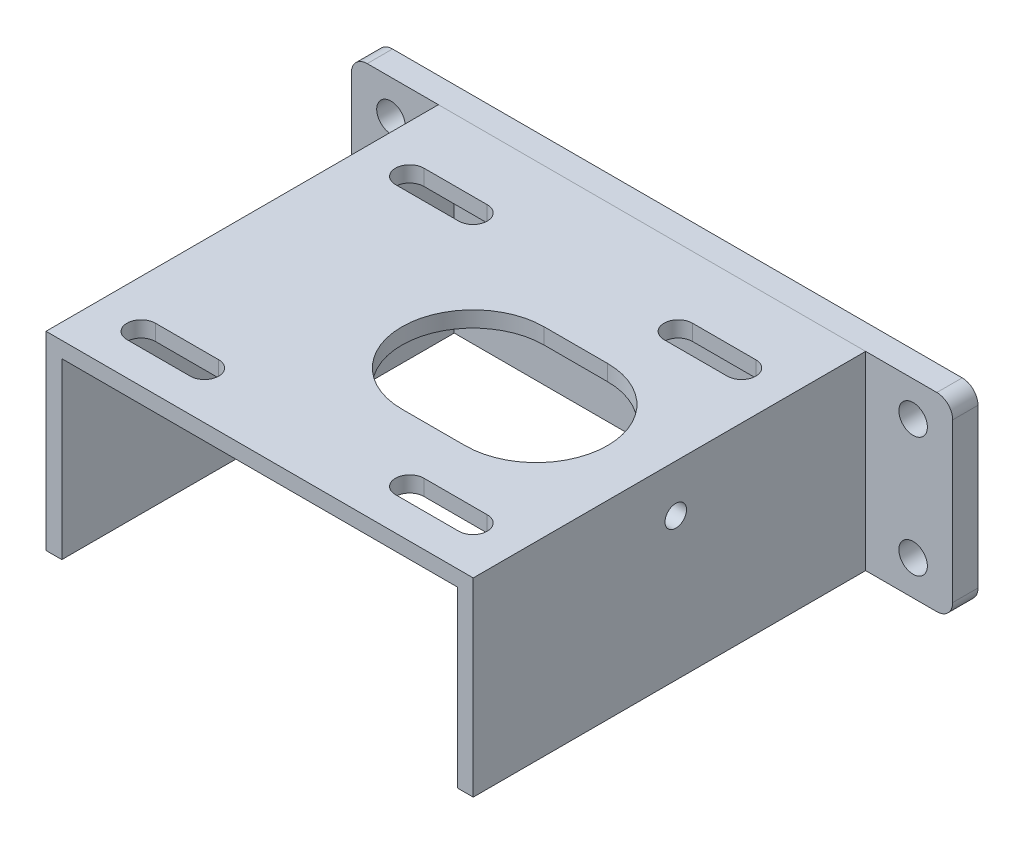
SolidWorks part; units mm, degrees
ref_plane "前视基准面" through (0, 0, 0) normal (0, 0, 1) x (1, 0, 0)
ref_plane "上视基准面" through (0, 0, 0) normal (0, 1, 0) x (1, 0, 0)
ref_plane "右视基准面" through (0, 0, 0) normal (1, 0, 0) x (0, 0, -1)
sketch "草图1" plane through (0, 0, 0) normal (0, 0, 1) x (1, 0, 0)
  line L1 (-95, 30) -> (95, 30)
  line L2 (-95, 30) -> (-95, -30)
  line L3 (-95, -30) -> (95, -30)
  line L4 (95, 30) -> (95, -30)
  line L5 (-95, 30) -> (95, -30) construction
  line L6 (-95, -30) -> (95, 30) construction
  point P0 (0, 0)
  dimension "D1" = 60
  dimension "D2" = 190
extrude "凸台-拉伸1" add sketch "草图1" along normal blind 8
sketch "草图2" plane through (0, 0, 8) normal (0, 0, 1) x (1, 0, 0)
  line L6 (-82.5, 19) -> (82.5, 19) construction
  line L7 (-82.5, 19) -> (-82.5, -19) construction
  line L8 (-82.5, -19) -> (82.5, -19) construction
  line L9 (82.5, 19) -> (82.5, -19) construction
  line L10 (-82.5, 19) -> (82.5, -19) construction
  line L11 (-82.5, -19) -> (82.5, 19) construction
  circle A0 centre (-82.5, 19) radius 4.5
  circle A1 centre (82.5, 19) radius 4.5
  circle A2 centre (82.5, -19) radius 4.5
  circle A3 centre (-82.5, -19) radius 4.5
  point P0 (0, 0)
  dimension "D3" = 9
  dimension "D1" = 165
  dimension "D2" = 38
extrude "切除-拉伸1" cut sketch "草图2" against normal blind 8
sketch "草图3" plane through (0, 0, 8) normal (0, 0, 1) x (1, 0, 0)
  line L0 (-67.5, 30) -> (-67.5, -30)
  line L1 (95, 30) -> (-95, 30) construction
  line L2 (-95, -30) -> (95, -30) construction
  line L3 (-67.5, -30) -> (-62.5, -30)
  line L4 (-62.5, -30) -> (-62.5, 25)
  line L5 (-62.5, 25) -> (62.5, 25)
  line L6 (62.5, 25) -> (62.5, -30)
  line L7 (62.5, -30) -> (67.5, -30)
  line L8 (67.5, -30) -> (67.5, 30)
  line L9 (67.5, 30) -> (-67.5, 30)
  line L10 (0, 0) -> (0, -46.5726) construction
  dimension "D1" = 5
  dimension "D2" = 5
  dimension "D3" = 135
extrude "凸台-拉伸2" add sketch "草图3" along normal blind 124 separate body
sketch "草图4" plane through (0, 30, 0) normal (0, 1, 0) x (1, 0, 0)
  line L0 (67.5, -132) -> (-67.5, -132) construction
  line L2 (0, -74.5736) -> (0, -132) construction
  line B0 (-32.4264, -112.5) -> (-52.4264, -112.5)
  line B1 (-32.4264, -36.6472) -> (-52.4264, -36.6472)
  arc B2 (-52.4264, -27.6472) -> (-52.4264, -36.6472) centre (-52.4264, -32.1472) ccw
  line B3 (-32.4264, -27.6472) -> (-52.4264, -27.6472)
  arc B4 (-32.4264, -36.6472) -> (-32.4264, -27.6472) centre (-32.4264, -32.1472) ccw
  line B5 (32.4264, -27.6472) -> (52.4264, -27.6472)
  arc B6 (52.4264, -36.6472) -> (52.4264, -27.6472) centre (52.4264, -32.1472) ccw
  line B7 (32.4264, -36.6472) -> (52.4264, -36.6472)
  arc B8 (32.4264, -27.6472) -> (32.4264, -36.6472) centre (32.4264, -32.1472) ccw
  line B9 (32.4264, -112.5) -> (52.4264, -112.5)
  arc B10 (52.4264, -121.5) -> (52.4264, -112.5) centre (52.4264, -117) ccw
  line B11 (32.4264, -121.5) -> (52.4264, -121.5)
  arc B12 (32.4264, -112.5) -> (32.4264, -121.5) centre (32.4264, -117) ccw
  line B13 (-32.4264, -121.5) -> (-52.4264, -121.5)
  arc B14 (-52.4264, -112.5) -> (-52.4264, -121.5) centre (-52.4264, -117) ccw
  arc B15 (-32.4264, -121.5) -> (-32.4264, -112.5) centre (-32.4264, -117) ccw
  line B16 (10, -52.0736) -> (30, -52.0736)
  arc B17 (30, -97.0736) -> (30, -52.0736) centre (30, -74.5736) ccw
  line B18 (10, -97.0736) -> (30, -97.0736)
  arc B19 (10, -52.0736) -> (10, -97.0736) centre (10, -74.5736) ccw
  line B20 (-32.4264, -32.1472) -> (-52.4264, -32.1472) construction
  line B21 (-42.4264, -117) -> (42.4264, -117) construction
  line B22 (42.4264, -117) -> (42.4264, -32.1472) construction
  dimension "D1" = 15
sketch_block_instance "调速电机60-90孔-2"
sketch_block "调速电机60-90孔" parameters "D6"=45, "D7"=9, "D1"=9, "D2"=15, "D3"=45, "D4"=120, "D5"=20, "D8"=84.8528
extrude "切除-拉伸2" cut sketch "草图4" against normal blind 150
fillet "圆角1" radius 5 4 edges at (95, -30, 4) (95, 30, 4) (-95, -30, 4) (-95, 30, 4)
sketch "草图5" plane through (67.5, 0, 0) normal (1, 0, 0) x (0, 0, -1)
  line L0 (-132, 30) -> (-8, 30) construction
  line L1 (-8, -30) -> (-8, 30) construction
  circle A0 centre (-68, 15) radius 3.4
  dimension "D1" = 6.8
  dimension "D2" = 15
  dimension "D3" = 60
extrude "切除-拉伸3" cut sketch "草图5" against normal through all
